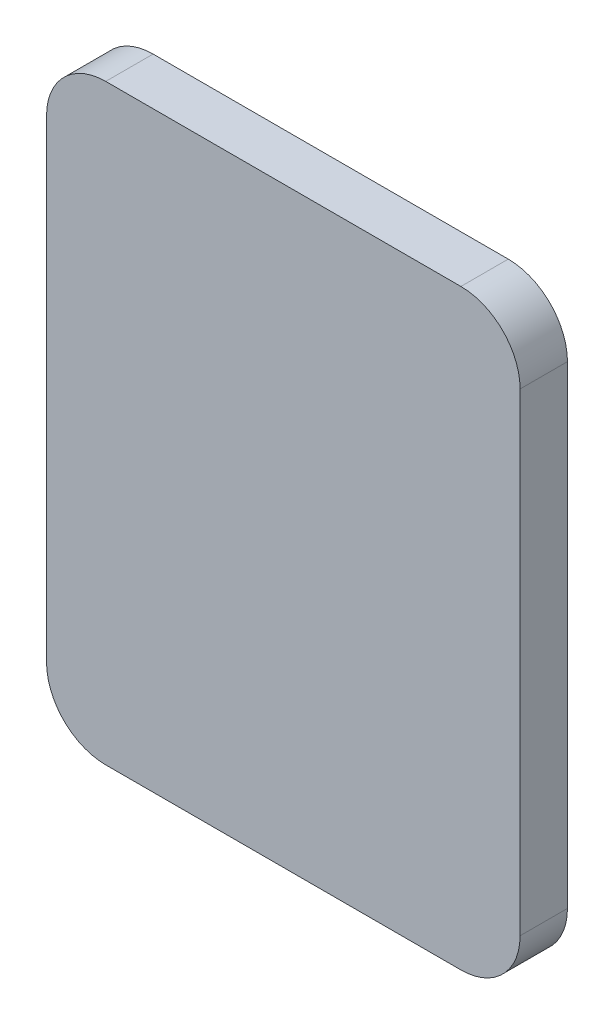
SolidWorks part; units mm, degrees
material "Q235"
ref_plane "Front Plane" through (0, 0, 0) normal (0, 0, 1) x (1, 0, 0)
ref_plane "Top Plane" through (0, 0, 0) normal (0, 1, 0) x (1, 0, 0)
ref_plane "Right Plane" through (0, 0, 0) normal (1, 0, 0) x (0, 0, -1)
sketch "Sketch1" plane through (0, 0, 0) normal (0, 0, 1) x (1, 0, 0)
  line L1 (10, 0) -> (70, 0)
  line L2 (0, 10) -> (0, 90)
  line L3 (10, 100) -> (70, 100)
  line L4 (80, 10) -> (80, 90)
  arc A0 (80, 90) -> (70, 100) centre (70, 90) ccw
  arc A1 (10, 100) -> (0, 90) centre (10, 90) ccw
  arc A2 (80, 10) -> (70, 0) centre (70, 10) cw
  arc A3 (10, 0) -> (0, 10) centre (10, 10) cw
  point P7 (80, 100)
  point P12 (80, 0)
  point P15 (0, 0)
  dimension "D3" = 10
  dimension "D4" = 10
  dimension "D1" = 80
  dimension "D2" = 100
extrude "Boss-Extrude1" add sketch "Sketch1" along normal blind 8
